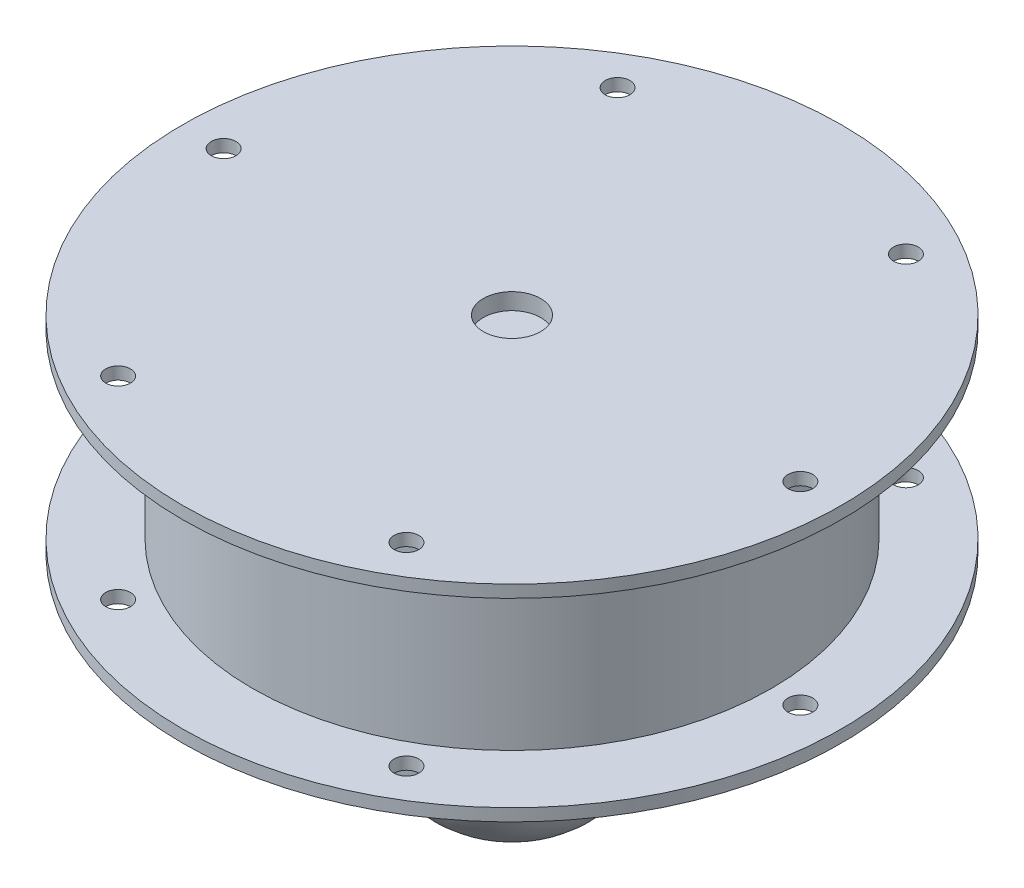
SolidWorks part; units mm, degrees
ref_plane "Front Plane" through (0, 0, 0) normal (0, 0, 1) x (1, 0, 0)
ref_plane "Top Plane" through (0, 0, 0) normal (0, 1, 0) x (1, 0, 0)
ref_plane "Right Plane" through (0, 0, 0) normal (1, 0, 0) x (0, 0, -1)
sketch "Sketch1" plane through (0, 0, 0) normal (0, 0, 1) x (1, 0, 0)
  line L0 (0, 0) -> (0, 43.0645) construction
  line L1 (-40, 0) -> (-30, 0)
  line L2 (-30, 0) -> (-30, 25)
  line L3 (-31.5, 1.5) -> (-31.5, 23.5)
  line L4 (-40, 1.5) -> (-31.5, 1.5)
  line L5 (-40, 1.5) -> (-40, 0)
  line L7 (-31.5, 23.5) -> (-40, 23.5)
  line L8 (-40, 23.5) -> (-40, 25)
  line L9 (-40, 25) -> (-30, 25)
  line L10 (-31.5, 1.5) -> (-31.5, 25) construction
  arc A2 (0, 55) -> (-30, 25) centre (0, 25) ccw construction
  arc A3 (0, 56.5) -> (-31.5, 25) centre (0, 25) ccw construction
  dimension "D2" = 1.5
  dimension "D1" = 10
  dimension "D3" = 30
  dimension "D4" = 25
  dimension "D6" = 40
  dimension "D5" = 1.5
revolve "Revolve1" add sketch "Sketch1" angle 360 about L0
sketch "Sketch2" plane through (0, 25, 0) normal (0, 1, 0) x (1, 0, 0)
  circle A0 centre (0, 0) radius 35 construction
  circle A1 centre (-35, 0) radius 1.5
  circle A2 centre (-17.5, 30.3109) radius 1.5
  circle A3 centre (17.5, 30.3109) radius 1.5
  circle A4 centre (35, 0) radius 1.5
  circle A5 centre (17.5, -30.3109) radius 1.5
  circle A6 centre (-17.5, -30.3109) radius 1.5
  point P18 (0, 0)
  dimension "D1" = 70
  dimension "D2" = 3
  dimension "D3" = 6
extrude "Cut-Extrude1" cut sketch "Sketch2" against normal through all
sketch "Sketch3" plane through (0, 25, 0) normal (0, 1, 0) x (1, 0, 0)
  circle A0 centre (0, 0) radius 30
extrude "Boss-Extrude1" add sketch "Sketch3" against normal blind 2
sketch "Sketch4" plane through (0, 23, 0) normal (0, -1, 0) x (-1, 0, 0)
  circle A0 centre (0, 0) radius 3.482
extrude "Cut-Extrude2" cut sketch "Sketch4" against normal blind 2
sketch "Sketch5" plane through (0, 23, 0) normal (0, -1, 0) x (-1, 0, 0)
  circle A0 centre (0, 0) radius 17.5
  dimension "D1" = 35
extrude "Boss-Extrude2" add sketch "Sketch5" along normal blind 35
sketch "Sketch6" plane through (0, -12, 0) normal (0, -1, 0) x (-1, 0, 0)
  circle A0 centre (0, 0) radius 13
  dimension "D1" = 26
extrude "Boss-Extrude3" add sketch "Sketch6" along normal blind 15
fillet "Fillet1" radius 12 1 edges at (0, -27, -13)
